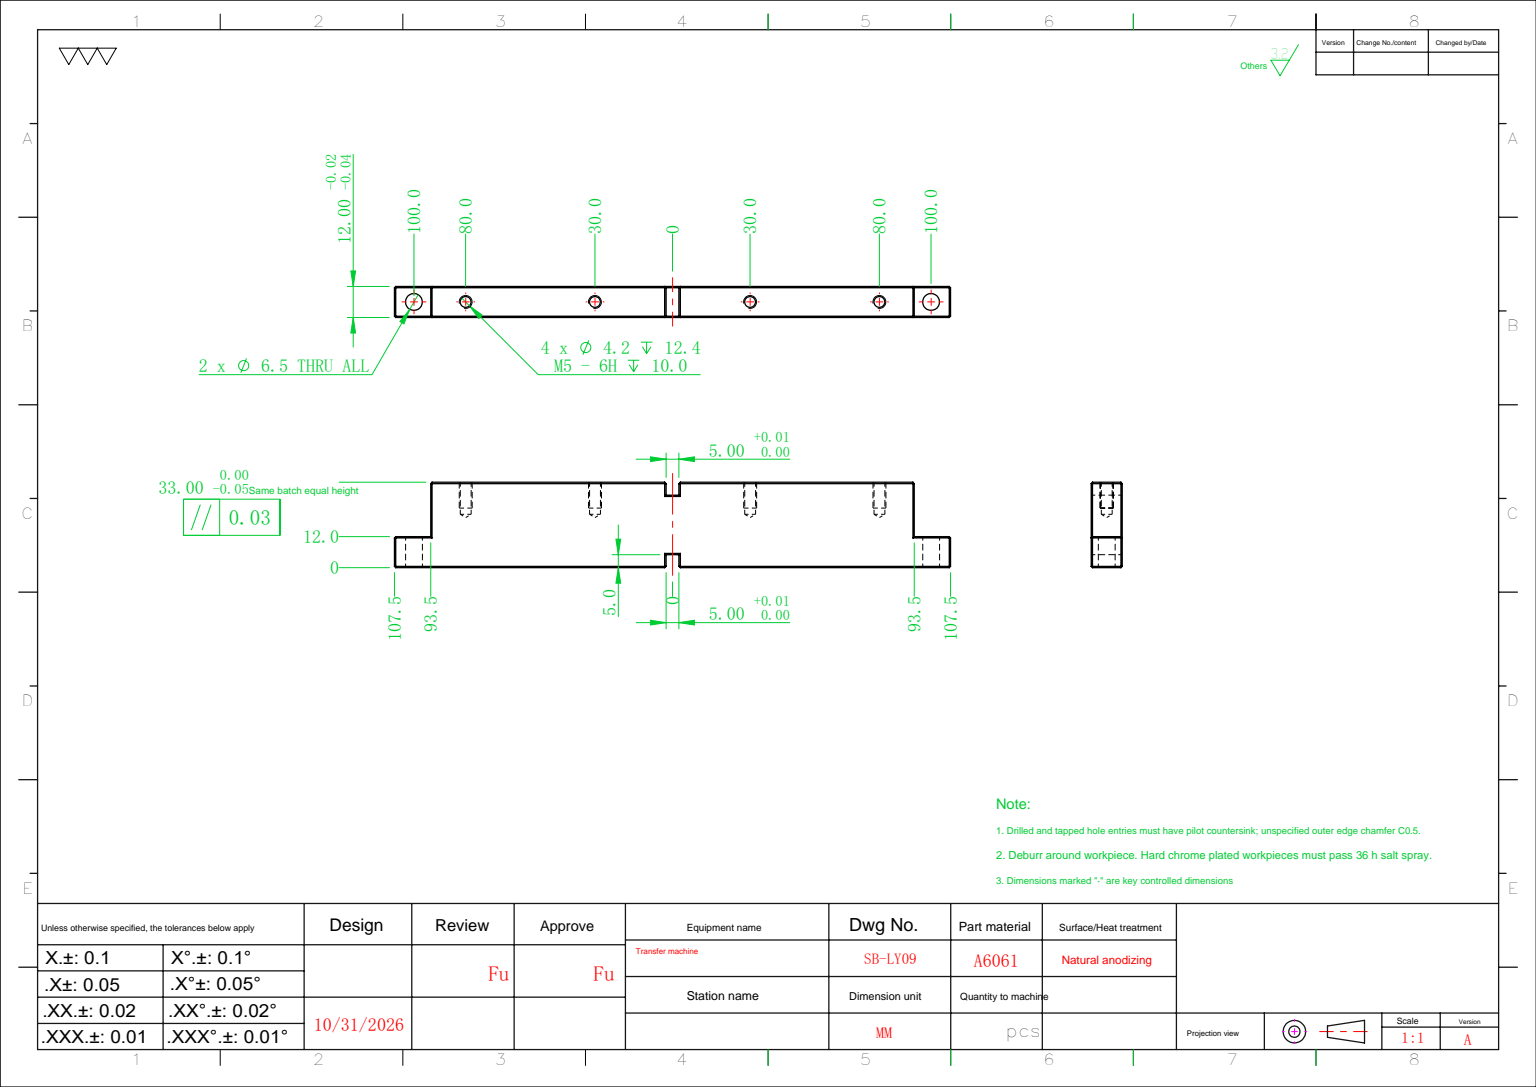
from build123d import *

# Parameters (mm, degrees)
SKETCH_1_W              = 187
SKETCH_1_H              = 33
EXTRUDE_1_DEPTH         = 12
HOLE_WIZARD_M5_1_D      = 4.2
HOLE_WIZARD_M5_1_DEPTH  = 12.4
HOLE_WIZARD_M5_1_TIP    = 1.2618073
SKETCH_8_W              = 5
SKETCH_8_H              = 12
CUT_EXTRUDE_2_DEPTH     = 5
SKETCH_11_W             = 5
SKETCH_11_H             = 5
CUT_EXTRUDE_3_DEPTH     = 96.700052247
SKETCH_12_W             = 14
SKETCH_12_H             = 12
EXTRUDE_2_DEPTH         = 12
HOLE_WIZARD_6_5_6_5_1_D = 6.5
CHAMFER_1_SIZE          = 0.5


with BuildPart() as part:
    # 草图1 → 凸台-拉伸1 (new body)
    with BuildSketch(Plane.XY):
        Rectangle(SKETCH_1_W, SKETCH_1_H)
    extrude(amount=EXTRUDE_1_DEPTH)

    # M5 螺纹孔1
    with Locations(Plane(origin=(0, -16.5, 0), x_dir=(-1, 0, 0), z_dir=(0, -1, 0))):
        with Locations((-80, -6), (-30, -6), (30, -6), (80, -6)):
            Hole(HOLE_WIZARD_M5_1_D / 2, depth=HOLE_WIZARD_M5_1_DEPTH)
            with Locations((0, 0, -(HOLE_WIZARD_M5_1_DEPTH + HOLE_WIZARD_M5_1_TIP / 2))):  # 118° drill point
                Cone(0, HOLE_WIZARD_M5_1_D / 2, HOLE_WIZARD_M5_1_TIP, mode=Mode.SUBTRACT)

    # 草图8 → 切除-拉伸2 (cut)
    with BuildSketch(Plane.XZ.offset(16.5)):
        with Locations((0, 6)):
            Rectangle(SKETCH_8_W, SKETCH_8_H)
    extrude(amount=-CUT_EXTRUDE_2_DEPTH, mode=Mode.SUBTRACT)

    # 草图11 → 切除-拉伸3 (cut, through all)
    with BuildSketch(Plane.XY.offset(12)):
        with Locations((0, 14)):
            Rectangle(SKETCH_11_W, SKETCH_11_H)
    extrude(amount=-CUT_EXTRUDE_3_DEPTH, mode=Mode.SUBTRACT)

    # 草图12 → 凸台-拉伸2 (add)
    with BuildSketch(Plane.XY.offset(12)):
        with Locations((100.5, 10.5)):
            Rectangle(SKETCH_12_W, SKETCH_12_H)
        with Locations((-100.5, 10.5)):
            Rectangle(SKETCH_12_W, SKETCH_12_H)
    extrude(amount=-EXTRUDE_2_DEPTH)

    # Ø6.5 (6.5) 直径孔1 (through all)
    with Locations(Plane(origin=(0, 4.5, 0), x_dir=(-1, 0, 0), z_dir=(0, -1, 0))):
        with Locations((-100, -6), (100, -6)):
            Hole(HOLE_WIZARD_6_5_6_5_1_D / 2)

    # 倒角1
    chamfer_1_edges = [part.edges().sort_by_distance(p)[0] for p in [
        (-48, -16.5, 12),
        (48, -16.5, 0),
        (48, -16.5, 12),
        (-2.5, -14, 0),
        (0, -11.5, 12),
        (-2.5, -14, 12),
        (2.5, -14, 12),
        (0, -11.5, 0),
        (2.5, -14, 0),
        (-2.5, -16.5, 6),
        (2.5, -16.5, 6),
        (93.5, -6, 12),
        (-48, -16.5, 0),
        (-55, 16.5, 0),
        (-55, 16.5, 12),
        (-2.5, 14, 0),
        (55, 16.5, 0),
        (-2.5, 16.5, 6),
        (2.5, 14, 0),
        (2.5, 16.5, 6),
        (0, 11.5, 0),
        (-2.5, 14, 12),
        (0, 11.5, 12),
        (2.5, 14, 12),
        (93.5, -6, 0),
        (100.5, 4.5, 12),
        (107.5, 10.5, 12),
        (100.5, 4.5, 0),
        (107.5, 4.5, 6),
        (107.5, 10.5, 0),
        (107.5, 16.5, 6),
        (93.5, -16.5, 6),
        (-93.5, -16.5, 6),
        (-93.5, -6, 0),
        (-93.5, -6, 12),
        (-107.5, 10.5, 12),
        (-100.5, 4.5, 12),
        (-107.5, 10.5, 0),
        (-107.5, 4.5, 6),
        (-100.5, 4.5, 0),
        (-107.5, 16.5, 6),
        (55, 16.5, 12),
    ]]
    chamfer(chamfer_1_edges, length=CHAMFER_1_SIZE)


solid = part.part
